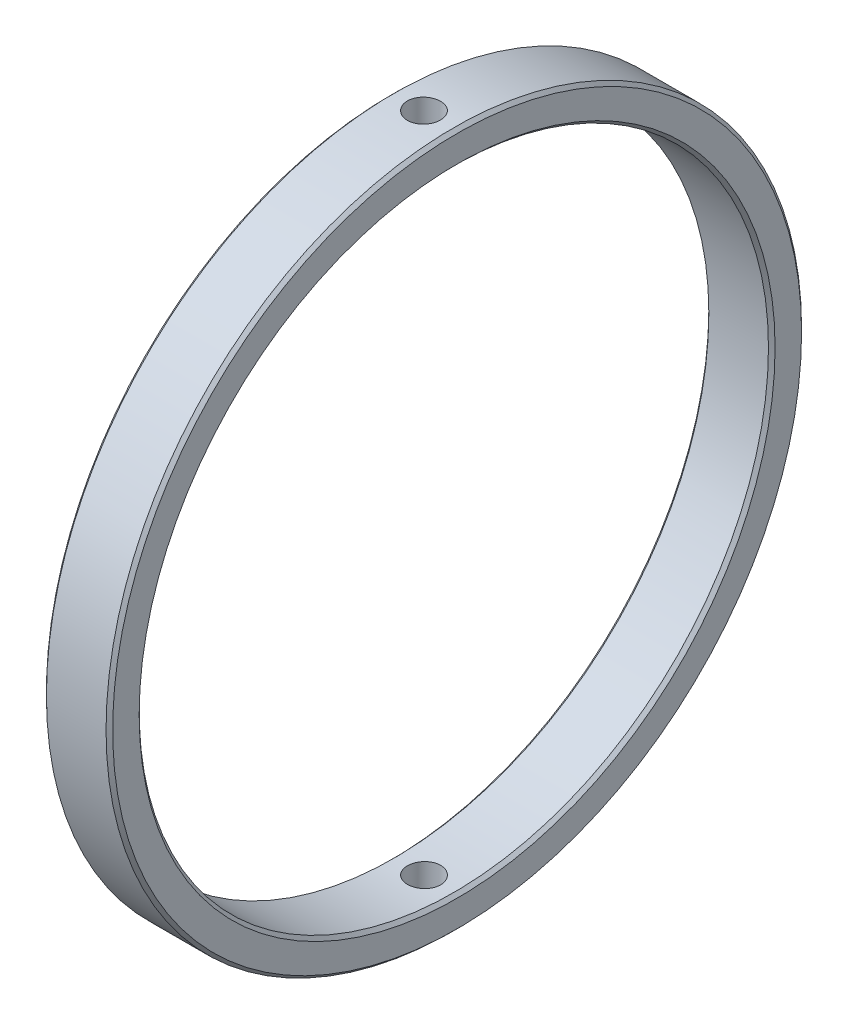
from build123d import *

# Parameters (mm, degrees)
SKETCH_1_R         = 52.5
SKETCH_1_R_2       = 47.5
EXTRUDE_1_DEPTH    = 5
CHAMFER_1_SIZE     = 0.5
HOLE_WIZARD_M6_1_D = 5


with BuildPart() as part:
    # 草图1 → 凸台-拉伸1 (new, symmetric)
    with BuildSketch(Plane(origin=(0, 0, 0), x_dir=(0, 0, -1), z_dir=(1, 0, 0))):
        Circle(SKETCH_1_R)
        Circle(SKETCH_1_R_2, mode=Mode.SUBTRACT)
    extrude(amount=EXTRUDE_1_DEPTH, both=True)

    # 倒角1
    chamfer_1_edges = [part.edges().sort_by_distance(p)[0] for p in [
        (-5, 0, 52.5),
        (5, 0, 52.5),
        (-5, 0, 47.5),
        (5, 0, 47.5),
    ]]
    chamfer(chamfer_1_edges, length=CHAMFER_1_SIZE)

    # M6 螺纹孔1 (through all)
    with Locations(Plane(origin=(0, 52.5, 0), x_dir=(1, 0, 0), z_dir=(0, 1, 0))):
        with Locations((0, 0)):
            Hole(HOLE_WIZARD_M6_1_D / 2)


solid = part.part
